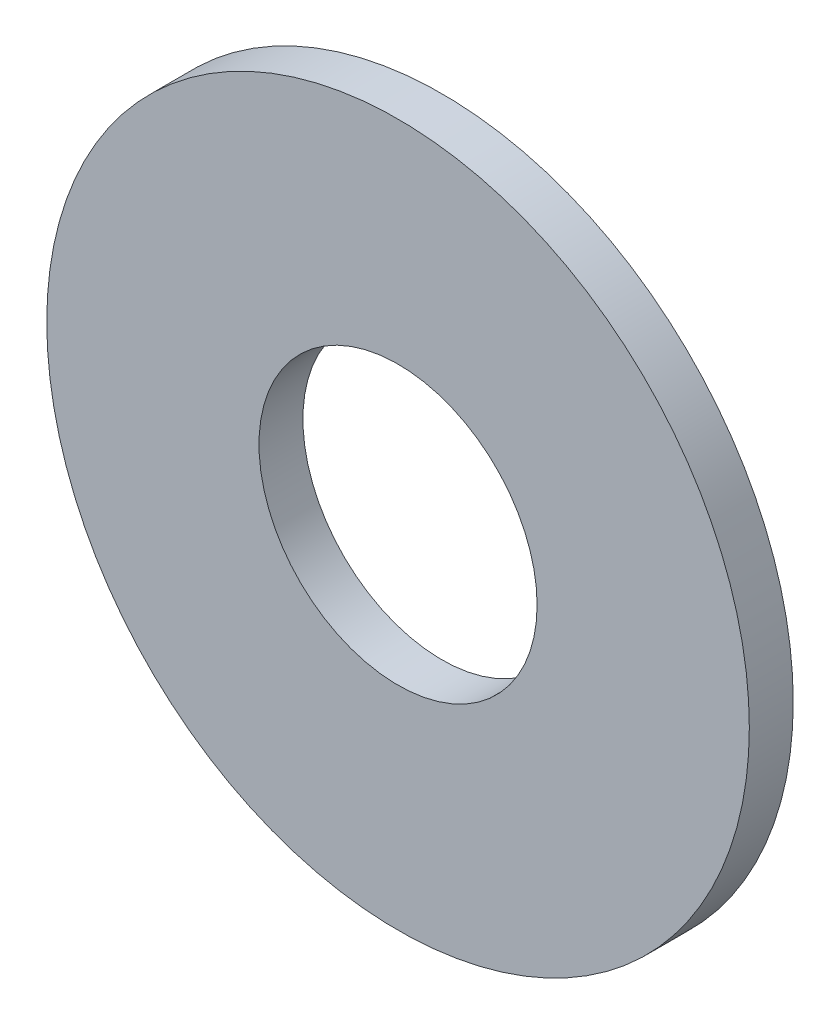
from build123d import *

# Parameters (mm, degrees)
SKETCH1_R      = 24
SKETCH1_R_2    = 9.5
EXTRUDE1_DEPTH = 3


with BuildPart() as part:
    # Sketch1 → Extrude1 (new body)
    with BuildSketch(Plane.XY):
        Circle(SKETCH1_R)
        Circle(SKETCH1_R_2, mode=Mode.SUBTRACT)
    extrude(amount=EXTRUDE1_DEPTH)


solid = part.part
